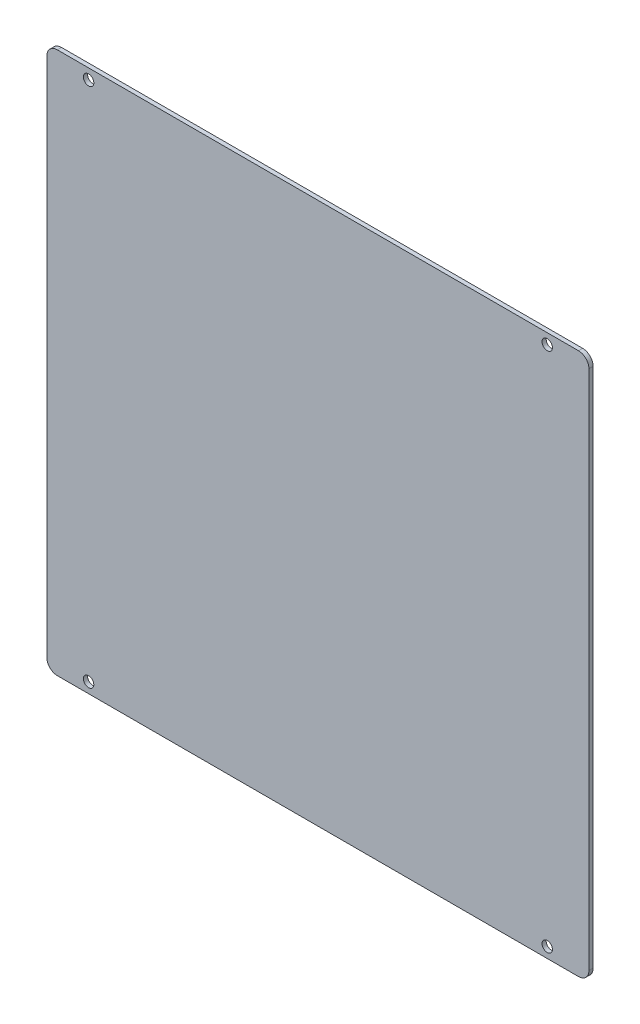
SolidWorks part; units mm, degrees
material "镀锌板"
ref_plane "前视基准面" through (0, 0, 0) normal (0, 0, 1) x (1, 0, 0)
ref_plane "上视基准面" through (0, 0, 0) normal (0, 1, 0) x (1, 0, 0)
ref_plane "右视基准面" through (0, 0, 0) normal (1, 0, 0) x (0, 0, -1)
sketch "草图1" plane through (0, 0, 0) normal (0, 0, 1) x (1, 0, 0)
  line L1 (-130, -130) -> (130, -130)
  line L2 (-130, -130) -> (-130, 130)
  line L3 (-130, 130) -> (130, 130)
  line L4 (130, -130) -> (130, 130)
  line L5 (-130, -130) -> (130, 130) construction
  line L6 (-130, 130) -> (130, -130) construction
  point P0 (0, 0)
  dimension "D1" = 260
  dimension "D2" = 260
extrude "凸台-拉伸1" add sketch "草图1" along normal blind 2
fillet "圆角1" radius 5 4 edges at (130, -130, 1) (-130, -130, 1) (-130, 130, 1) (130, 130, 1)
hole_wizard "Ø5.0 (5) 直径孔1" positions "草图2" profile "草图3" hole size "Ø5.0" standard "GB" end condition through all
sketch "草图2" plane through (0, 0, 2) normal (0, 0, 1) x (1, 0, 0)
  line L0 (-69.7215, 0) -> (0, 0) construction
  line L1 (0, 0) -> (0, 29.1857) construction
  point P0 (-110, 125)
  point P10 (-110, -125)
  point P11 (110, -125)
  point P12 (110, 125)
  dimension "D1" = 220
  dimension "D2" = 250
sketch "草图3" plane through (-110, 125, 2) normal (1, 0, 0) x (0, -1, 0)
  line L0 (0, 0) -> (0, 2)
  line L1 (0, 2) -> (2.5, 2)
  line L2 (2.5, 2) -> (2.5, 0)
  line L5 (2.5, 0) -> (0, 0)
  line L11 (0, -6.35) -> (0, 107.95) construction
  dimension "通孔孔直径" = 5
  dimension "通孔孔深度" = 2
